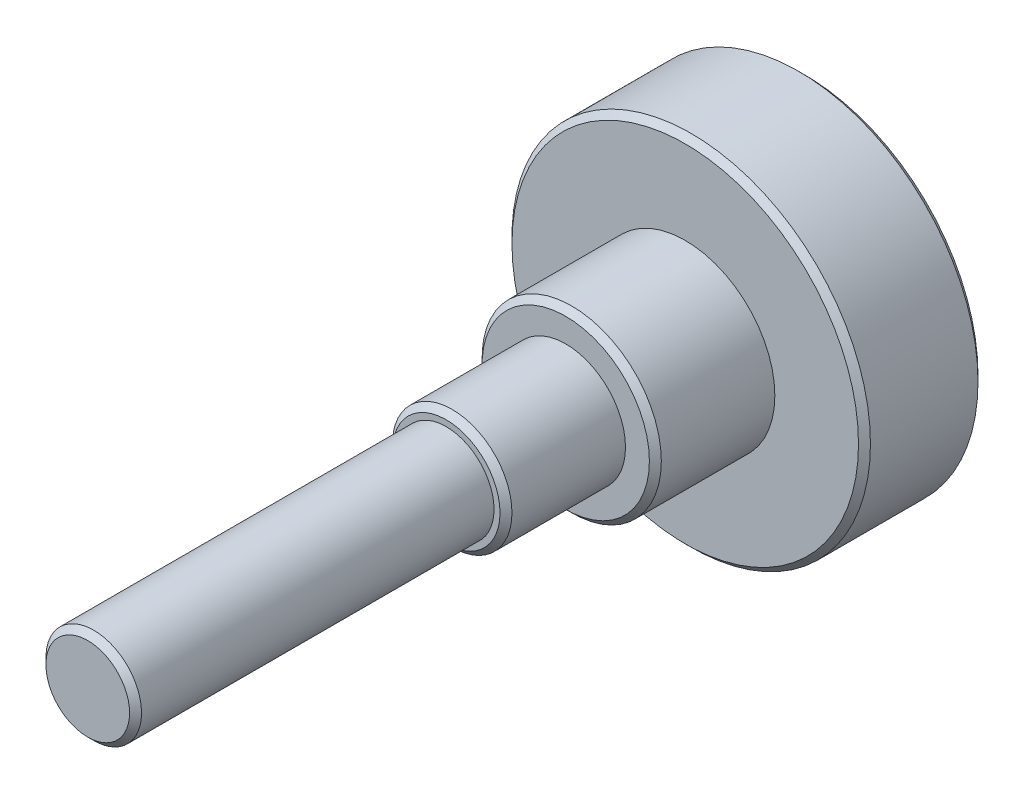
SolidWorks part; units mm, degrees
material "S45C"
ref_plane "Front Plane" through (0, 0, 0) normal (0, 0, 1) x (1, 0, 0)
ref_plane "Top Plane" through (0, 0, 0) normal (0, 1, 0) x (1, 0, 0)
ref_plane "Right Plane" through (0, 0, 0) normal (1, 0, 0) x (0, 0, -1)
sketch "Sketch1" plane through (0, 0, 0) normal (0, 0, 1) x (1, 0, 0)
  circle A0 centre (0, 0) radius 15
  dimension "D1" = 30
extrude "Boss-Extrude1" add sketch "Sketch1" along normal blind 10
sketch "Sketch2" plane through (0, 0, 10) normal (0, 0, 1) x (1, 0, 0)
  circle A0 centre (0, 0) radius 7.5
  dimension "D1" = 15
extrude "Boss-Extrude2" add sketch "Sketch2" along normal blind 10
sketch "Sketch3" plane through (0, 0, 20) normal (0, 0, 1) x (1, 0, 0)
  circle A0 centre (0, 0) radius 4
  dimension "D1" = 8
extrude "Boss-Extrude3" add sketch "Sketch3" along normal blind 40
cosmetic thread "Cosmetic Thread1" parameters "D1"=30, "D2"=6.891
sketch "Sketch4" plane through (0, 0, 20) normal (0, 0, 1) x (1, 0, 0)
  circle A0 centre (0, 0) radius 5
  dimension "D1" = 10
extrude "Boss-Extrude4" add sketch "Sketch4" along normal blind 10
chamfer "Chamfer1" distance 0.5 angle 45 5 edges at (15, 0, 0) (15, 0, 10) (7.5, 0, 20) (5, 0, 30) (4, 0, 60)
